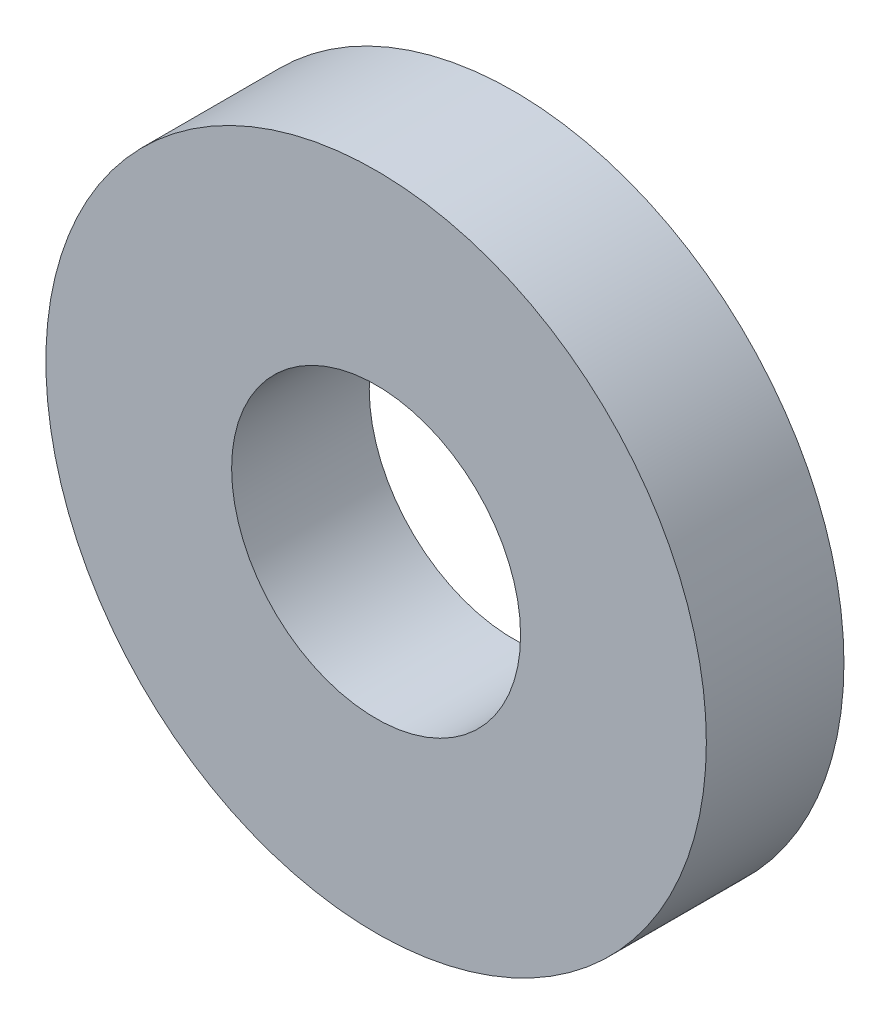
from build123d import *

# Parameters (mm, degrees)
SKETCH1_R           = 12
SKETCH1_R_2         = 5.25
BOSS_EXTRUDE1_DEPTH = 5


with BuildPart() as part:
    # Sketch1 → Boss-Extrude1 (new body)
    with BuildSketch(Plane.XY):
        Circle(SKETCH1_R)
        Circle(SKETCH1_R_2, mode=Mode.SUBTRACT)
    extrude(amount=BOSS_EXTRUDE1_DEPTH)


solid = part.part
